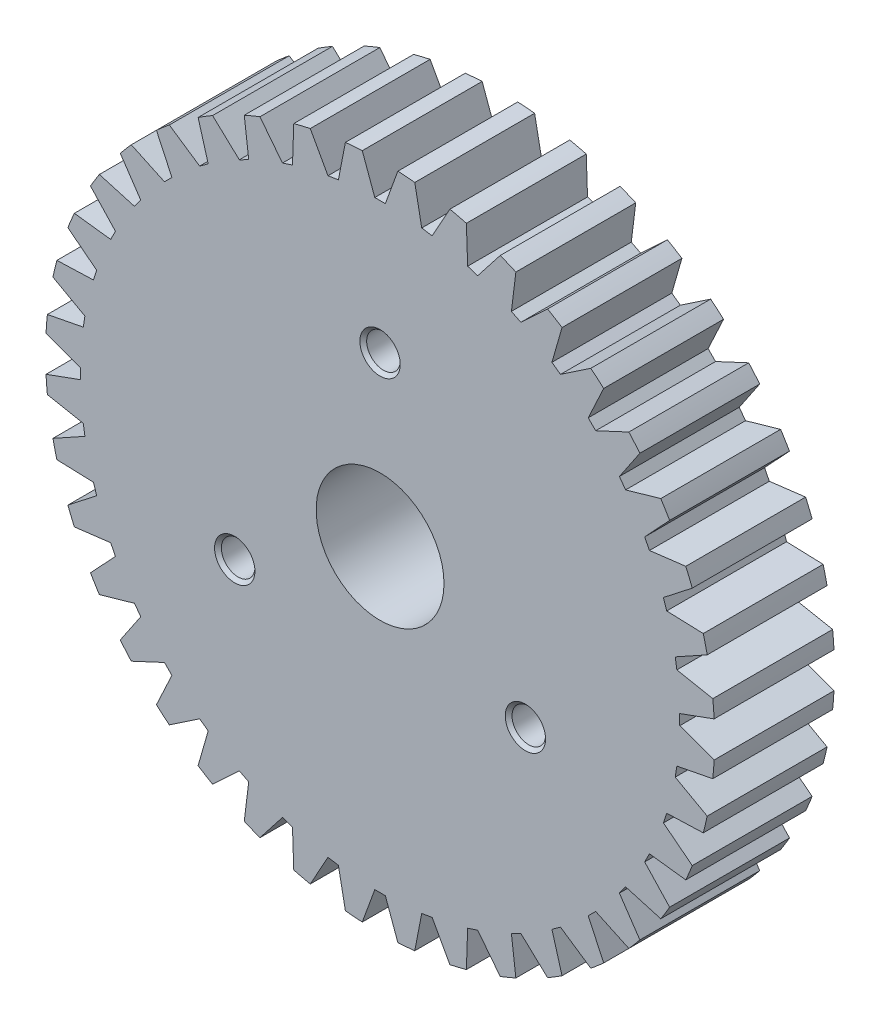
SolidWorks part; units mm, degrees
ref_plane "Front Plane" through (0, 0, 0) normal (0, 0, 1) x (1, 0, 0)
ref_plane "Top Plane" through (0, 0, 0) normal (0, 1, 0) x (1, 0, 0)
ref_plane "Right Plane" through (0, 0, 0) normal (1, 0, 0) x (0, 0, -1)
other "Configuration Table"
sketch "Sketch1" plane through (0, 0, 0) normal (0, 0, 1) x (1, 0, 0)
  circle A0 centre (0, 0) radius 8
  circle A1 centre (0, 0) radius 41.86
  dimension "D1" = 83.72
  dimension "D2" = 16
extrude "Boss-Extrude1" add sketch "Sketch1" along normal blind 15
sketch "Sketch2" plane through (0, 0, 15) normal (0, 0, 1) x (1, 0, 0)
  circle A0 centre (0, 0) radius 21 construction
  point P6 (0, 21)
  point P12 (18.1865, -10.5)
  point P13 (-18.1865, -10.5)
  dimension "D1" = 42
  dimension "D2" = 3
hole_wizard "M5 Tapped Hole1" positions "Sketch2" profile "Sketch3" tap size "M5" standard "GB"
sketch "Sketch3" plane through (-18.1865, -10.5, 15) normal (1, 0, 0) x (0, -1, 0)
  line L0 (0, 0) -> (0, 11.2618)
  line L1 (0, 11.2618) -> (2.1, 10)
  line L2 (2.1, 10) -> (2.1, 0.425)
  line L3 (2.1, 0.425) -> (2.525, 0)
  line L5 (2.525, 0) -> (0, 0)
  line L6 (-2.1, 0.425) -> (-2.525, 0) construction
  line L10 (0, 11.2618) -> (-2.1, 10) construction
  line L11 (0, -6.35) -> (0, 107.95) construction
  dimension "螺纹孔钻头直径" = 4.2
  dimension "螺纹孔钻头深度" = 10
  dimension "近端锥形沉头孔直径" = 5.05
  dimension "近端锥形沉头孔角度" = 90
  dimension "导头角度" = 118
cosmetic thread "Hole cosmetic thread 1" parameters "D1"=8, "D2"=5
cosmetic thread "Hole cosmetic thread 2" parameters "D1"=8, "D2"=5
cosmetic thread "Hole cosmetic thread 3" parameters "D1"=8, "D2"=5
sketch "Sketch4" plane through (0, 0, 0) normal (0, 0, 1) x (1, 0, 0)
  line L0 (0, 49.3244) -> (0, 0) construction
  line L1 (0.6601, 37.5) -> (-0.6601, 37.5)
  line L2 (-0.6601, 37.5) -> (-3.8576, 46.285)
  line L3 (-3.8576, 46.285) -> (3.8576, 46.285)
  line L4 (-1.57, 40) -> (1.57, 40) construction
  line L5 (0.6601, 37.5) -> (3.8576, 46.285)
  point P10 (0, 40)
  point P11 (0, 46.285)
  point P12 (0, 37.5)
  dimension "D1" = 20
  dimension "D2" = 40
  dimension "D3" = 3.14
  dimension "D4" = 2.5
extrude "Cut-Extrude1" cut sketch "Sketch4" along normal blind 15
pattern_circular "CirPattern1" count 40 over 360 about axis through (0, 0, 0) along (0, 0, 1) of "Cut-Extrude1"
